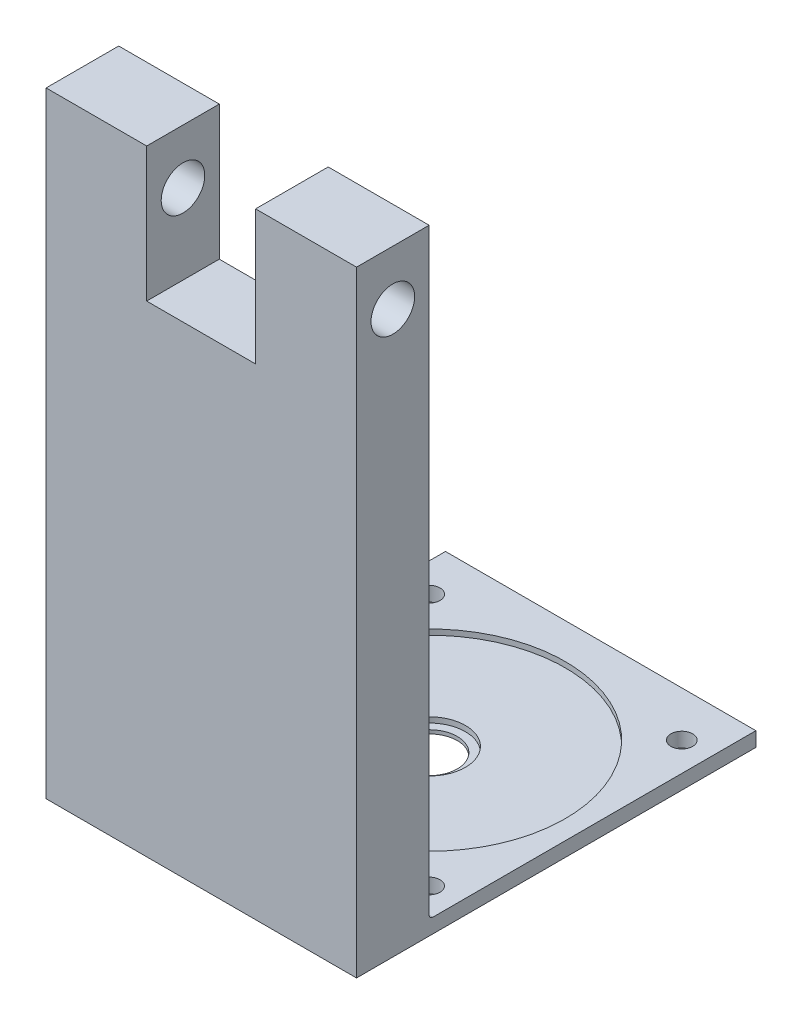
from build123d import *

# Parameters (mm, degrees)
EXTRUDE_1_DEPTH          = 20
SKETCH_2_W               = 30
SKETCH_2_H               = 37
CUT_EXTRUDE_1_DEPTH      = 20
CUT_EXTRUDE_2_DEPTH      = 157.04887055
CUT_EXTRUDE_2_DEPTH_BACK = 157.04887055
SKETCH_3_R               = 6
CUT_EXTRUDE_3_DEPTH      = 138.362886181
CUT_EXTRUDE_3_DEPTH_BACK = 138.362886181
SKETCH_4_W               = 85.5
SKETCH_4_H               = 10
SKETCH_5_W               = 85.5
SKETCH_5_H               = 20
CUT_EXTRUDE_4_DEPTH      = 8.43
EXTRUDE_START            = -20
SKETCH_6_W               = 85.5
SKETCH_6_H               = 4
EXTRUDE_2_DEPTH          = 90
SKETCH_8_R               = 3
CUT_EXTRUDE_6_DEPTH      = 90
FILLET_1_R               = 1
SKETCH_9_R               = 37.5
CUT_EXTRUDE_7_DEPTH      = 1.5
CUT_EXTRUDE_8_DEPTH      = 195.524927451
CUT_EXTRUDE_8_DEPTH_BACK = 195.524927451
SKETCH_10_R              = 7.75
SKETCH_11_R              = 10
CUT_EXTRUDE_9_DEPTH      = 1.5


with BuildPart() as part:
    # 草图1 → 凸台-拉伸1 (new body)
    with BuildSketch(Plane.XY):
        Polygon((-42.75, -59), (-42.75, 59), (-42.75, 129), (42.75, 129), (42.75, 59), (42.75, -59), align=None)
    extrude(amount=EXTRUDE_1_DEPTH)

    # 草图2 → 切除-拉伸1 (cut)
    with BuildSketch(Plane.XY.offset(20)):
        with Locations((-0.051962385, 110.5)):
            Rectangle(SKETCH_2_W, SKETCH_2_H)
    extrude(amount=-CUT_EXTRUDE_1_DEPTH, mode=Mode.SUBTRACT)

    # 草图3 → 切除-拉伸2 (cut, two sides: drawn at the far end of the back side and taken through both)
    with BuildSketch(Plane.ZY.offset(42.75).offset(-CUT_EXTRUDE_2_DEPTH_BACK)):
        with Locations((10, 114)):
            Circle(SKETCH_3_R)
    extrude(amount=CUT_EXTRUDE_2_DEPTH + CUT_EXTRUDE_2_DEPTH_BACK, mode=Mode.SUBTRACT)

    # 草图4 → 切除-拉伸3 (cut, two sides: drawn at the far end of the back side and taken through both)
    with BuildSketch(Plane.XY.offset(20).offset(-CUT_EXTRUDE_3_DEPTH_BACK)):
        with Locations((0, -54)):
            Rectangle(SKETCH_4_W, SKETCH_4_H)
    extrude(amount=CUT_EXTRUDE_3_DEPTH + CUT_EXTRUDE_3_DEPTH_BACK, mode=Mode.SUBTRACT)

    # 草图5 → 切除-拉伸4 (cut)
    with BuildSketch(Plane.XZ.offset(49)):
        with Locations((0, 10)):
            Rectangle(SKETCH_5_W, SKETCH_5_H)
    extrude(amount=-CUT_EXTRUDE_4_DEPTH, mode=Mode.SUBTRACT)

    # 草图6 → 凸台-拉伸2 (add)
    with BuildSketch(Plane.XY.offset(20).offset(EXTRUDE_START)):
        with Locations((0, -38.57)):
            Rectangle(SKETCH_6_W, SKETCH_6_H)
    extrude(amount=-EXTRUDE_2_DEPTH)

    # 草图8 → 切除-拉伸6 (cut)
    with BuildSketch(Plane(origin=(0, -36.57, 0), x_dir=(1, 0, 0), z_dir=(0, 1, 0))):
        with Locations(Location((-34.8, 77.55, 0), (0, 0, 270))):
            Circle(SKETCH_8_R)
        with Locations(Location((34.8, 77.55, 0), (0, 0, 270))):
            Circle(SKETCH_8_R)
        with Locations(Location((-34.8, 7.95, 0), (0, 0, 270))):
            Circle(SKETCH_8_R)
        with Locations(Location((34.8, 7.95, 0), (0, 0, 270))):
            Circle(SKETCH_8_R)
    extrude(amount=-CUT_EXTRUDE_6_DEPTH, mode=Mode.SUBTRACT)

    # 圆角1
    fillet_1_edges = [part.edges().sort_by_distance(p)[0] for p in [
        (0, -36.57, 0),
    ]]
    fillet(fillet_1_edges, radius=FILLET_1_R)

    # 草图9 → 切除-拉伸7 (cut)
    with BuildSketch(Plane(origin=(0, -36.57, 0), x_dir=(1, 0, 0), z_dir=(0, 1, 0))):
        with Locations(Location((0, 42.75, 0), (0, 0, 270))):
            Circle(SKETCH_9_R)
    extrude(amount=-CUT_EXTRUDE_7_DEPTH, mode=Mode.SUBTRACT)

    # 草图10 → 切除-拉伸8 (cut, two sides: drawn at the far end of the back side and taken through both)
    with BuildSketch(Plane(origin=(0, -38.07, 0), x_dir=(1, 0, 0), z_dir=(0, 1, 0)).offset(-CUT_EXTRUDE_8_DEPTH_BACK)):
        with Locations(Location((0, 42.75, 0), (0, 0, 270))):
            Circle(SKETCH_10_R)
    extrude(amount=CUT_EXTRUDE_8_DEPTH + CUT_EXTRUDE_8_DEPTH_BACK, mode=Mode.SUBTRACT)

    # 草图11 → 切除-拉伸9 (cut)
    with BuildSketch(Plane(origin=(0, -38.07, 0), x_dir=(1, 0, 0), z_dir=(0, 1, 0))):
        with Locations(Location((0, 42.75, 0), (0, 0, 270))):
            Circle(SKETCH_11_R)
    extrude(amount=-CUT_EXTRUDE_9_DEPTH, mode=Mode.SUBTRACT)


solid = part.part
